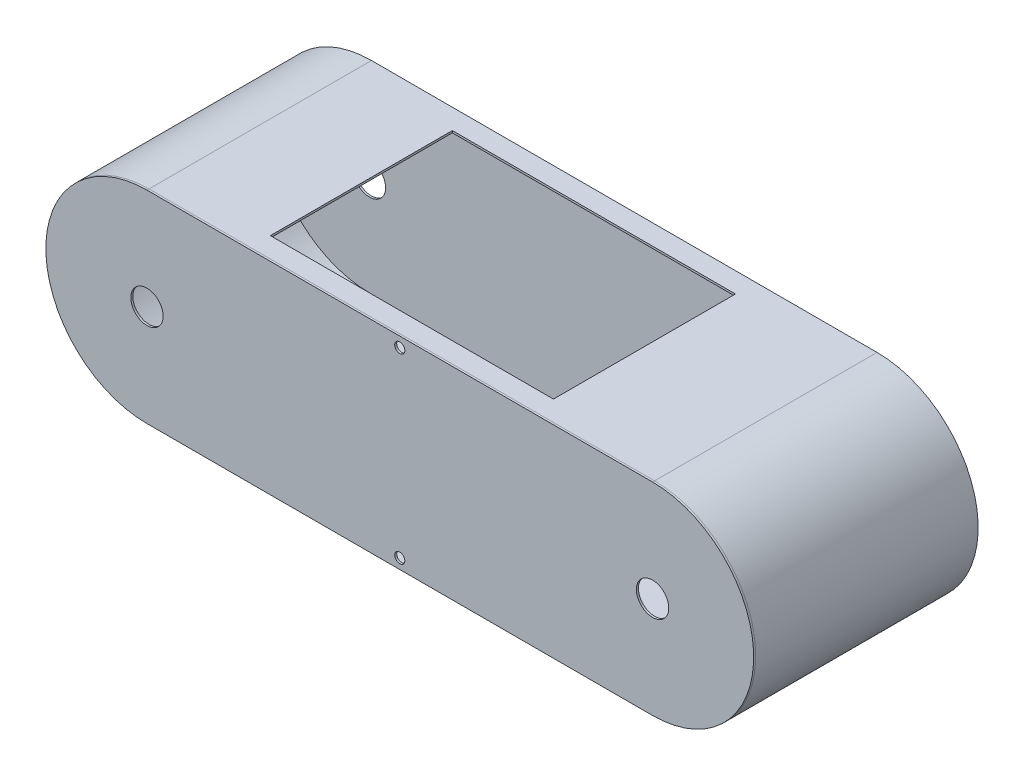
SolidWorks part; units mm, degrees
ref_plane "前视基准面" through (0, 0, 0) normal (0, 0, 1) x (1, 0, 0)
ref_plane "上视基准面" through (0, 0, 0) normal (0, 1, 0) x (1, 0, 0)
ref_plane "右视基准面" through (0, 0, 0) normal (1, 0, 0) x (0, 0, -1)
sketch "草图1" plane through (0, 0, 0) normal (0, 0, 1) x (1, 0, 0)
  line L0 (0, 0) -> (250, 0) construction
  line L1 (0, 50) -> (250, 50)
  line L2 (0, -50) -> (250, -50)
  arc A0 (0, 50) -> (0, -50) centre (0, 0) ccw
  arc A1 (250, -50) -> (250, 50) centre (250, 0) ccw
  point P3 (125, 0)
  dimension "D1" = 50
  dimension "D2" = 250
extrude "凸台-拉伸1" add sketch "草图1" along normal blind 110
shell "抽壳1" thickness 1
sketch "草图2" plane through (0, 0, 110) normal (0, 0, 1) x (1, 0, 0)
  line L0 (0, -50) -> (250, -50) construction
  line L1 (250, 50) -> (0, 50) construction
  line L2 (0, -50) -> (250, -50)
  line L3 (250, 50) -> (0, 50)
  arc A0 (250, -50) -> (250, 50) centre (250, 0) ccw construction
  arc A1 (0, 50) -> (0, -50) centre (0, 0) ccw construction
  arc A2 (250, -50) -> (250, 50) centre (250, 0) ccw
  arc A3 (0, 50) -> (0, -50) centre (0, 0) ccw
extrude "凸台-拉伸2" add sketch "草图2" along normal blind 1 separate body
sketch "草图3" plane through (0, 0, 111) normal (0, 0, 1) x (1, 0, 0)
  circle A0 centre (0, 0) radius 8
  circle A1 centre (250, 0) radius 8
  dimension "D1" = 16
extrude "切除-拉伸1" cut sketch "草图3" against normal through all
sketch "草图4" plane through (0, -50, 0) normal (0, -1, 0) x (1, 0, 0)
  line L0 (0, 55) -> (250, 55) construction
  line L1 (0, 110) -> (0, 0) construction
  line L2 (250, 110) -> (250, 0) construction
sketch "草图5" plane through (0, 0, 111) normal (0, 0, 1) x (1, 0, 0)
  line L0 (125, 50) -> (125, -50) construction
  line L1 (250, 50) -> (0, 50) construction
  line L2 (0, -50) -> (250, -50) construction
  line L3 (125, 0) -> (639.2914, 0) construction
  circle A0 centre (-100, 45) radius 2.5
  circle A1 centre (350, 45) radius 2.5
  circle A2 centre (-100, -45) radius 2.5
  circle A3 centre (350, -45) radius 2.5
  circle A4 centre (420, 0) radius 2.5
  circle A5 centre (-170, 0) radius 2.5
  circle A6 centre (125, 45) radius 2.5
  circle A7 centre (125, -45) radius 2.5
  dimension "D1" = 5
  dimension "D2" = 450
  dimension "D3" = 5
  dimension "D4" = 590
extrude "切除-拉伸2" cut sketch "草图5" against normal blind 3
sketch "草图6" plane through (0, -50, 0) normal (0, -1, 0) x (1, 0, 0)
  line L0 (125, 110) -> (125, 0) construction
  line L1 (0, 110) -> (250, 110) construction
  line L2 (0, 0) -> (250, 0) construction
  line L3 (0, 55) -> (250, 55) construction
  line L4 (55, 10) -> (135, 10)
  line L5 (55, 10) -> (55, 100)
  line L6 (55, 100) -> (135, 100)
  line L7 (135, 10) -> (135, 100)
  line L8 (55, 10) -> (135, 100) construction
  line L9 (55, 100) -> (135, 10) construction
  point P6 (95, 55)
  dimension "D1" = 80
  dimension "D2" = 90
  dimension "D3" = 10
extrude "切除-拉伸3" cut sketch "草图6" against normal blind 3
sketch "草图7" plane through (0, 50, 0) normal (0, 1, 0) x (1, 0, 0)
  line L0 (0, -55) -> (250, -55) construction
  line L1 (50, -100) -> (190, -100)
  line L2 (50, -100) -> (50, -10)
  line L3 (50, -10) -> (190, -10)
  line L4 (190, -100) -> (190, -10)
  line L5 (50, -100) -> (190, -10) construction
  line L6 (50, -10) -> (190, -100) construction
  line L7 (0, -110) -> (0, 0) construction
  point P0 (120, -55)
  dimension "D1" = 140
  dimension "D2" = 90
  dimension "D3" = 50
extrude "切除-拉伸4" cut sketch "草图7" against normal blind 3
